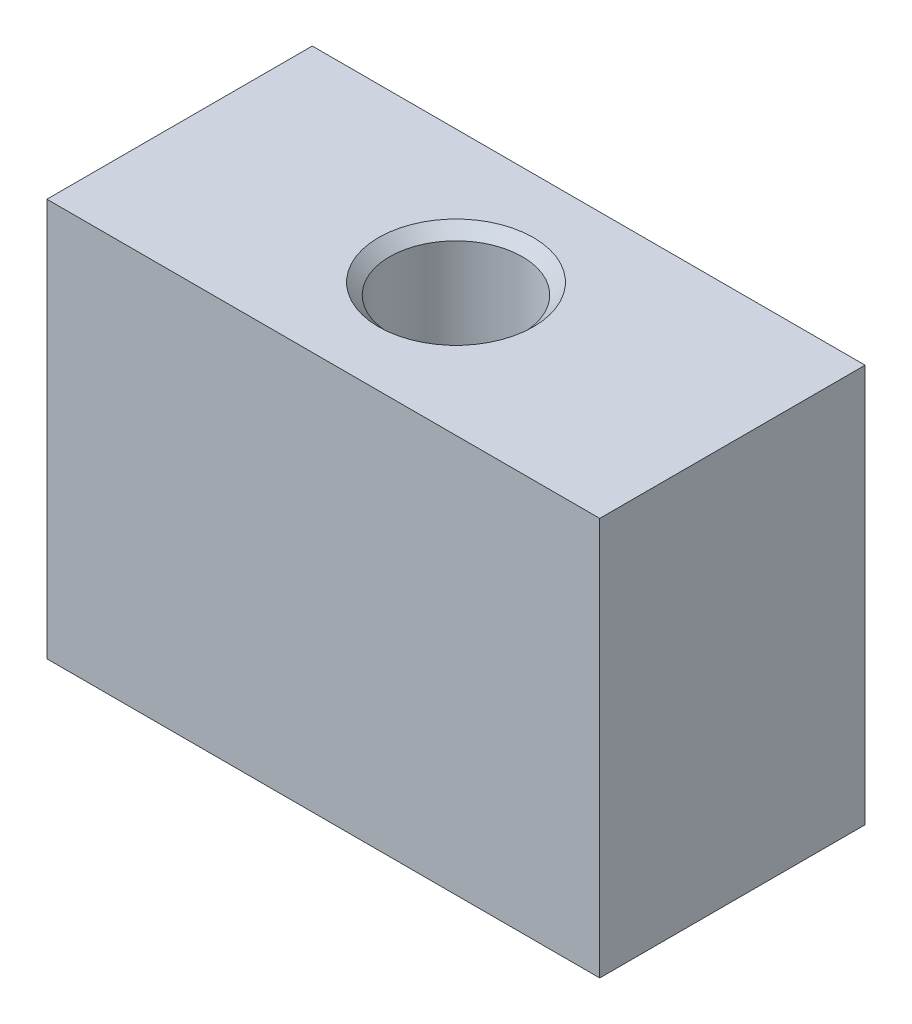
SolidWorks part; units mm, degrees
ref_plane "Front Plane" through (0, 0, 0) normal (0, 0, 1) x (1, 0, 0)
ref_plane "Top Plane" through (0, 0, 0) normal (0, 1, 0) x (1, 0, 0)
ref_plane "Right Plane" through (0, 0, 0) normal (1, 0, 0) x (0, 0, -1)
other "Configuration Table"
sketch "Sketch1" plane through (0, 0, 0) normal (0, 1, 0) x (1, 0, 0)
  line L1 (-12.5, -6) -> (12.5, -6)
  line L2 (-12.5, -6) -> (-12.5, 6)
  line L3 (-12.5, 6) -> (12.5, 6)
  line L4 (12.5, -6) -> (12.5, 6)
  line L5 (-12.5, -6) -> (12.5, 6) construction
  line L6 (-12.5, 6) -> (12.5, -6) construction
  point P0 (0, 0)
  dimension "D1" = 25
  dimension "D2" = 12
extrude "Boss-Extrude1" add sketch "Sketch1" along normal blind 18
sketch "Sketch2" plane through (0, 0, 0) normal (0, 1, 0) x (1, 0, 0)
  line L0 (12.5, 6) -> (-12.5, 6) construction
  circle A0 centre (0, 0) radius 3
  dimension "D1" = 6
  dimension "D2" = 6
extrude "Cut-Extrude1" cut sketch "Sketch2" along normal through all
chamfer "Chamfer1" distance 0.5 angle 45 2 edges at (0, 0, 3) (0, 18, 3)
